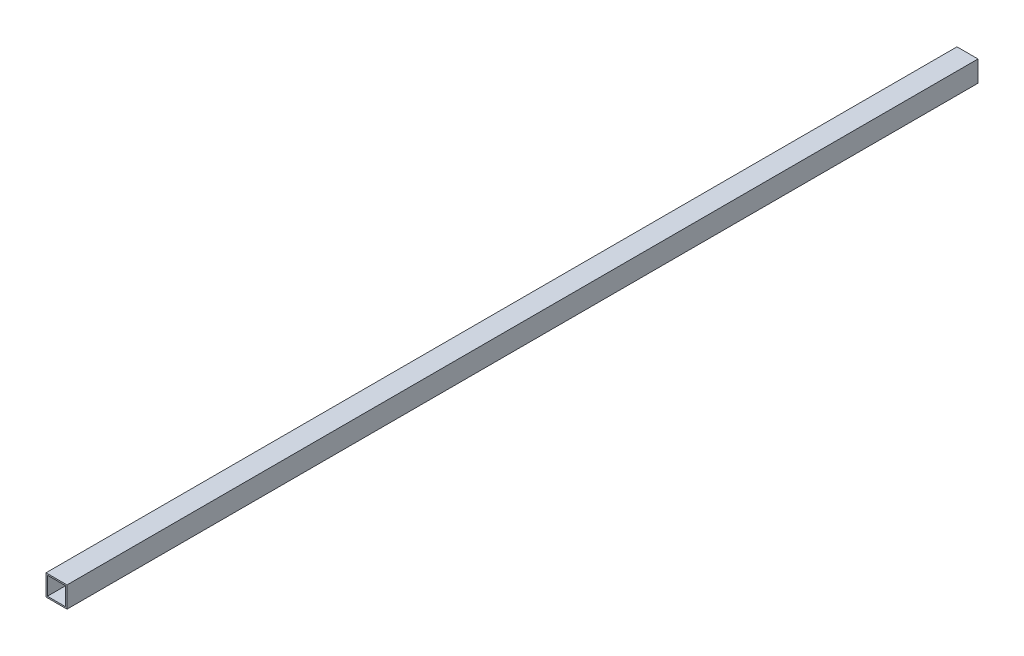
from build123d import *

# Parameters (mm, degrees)
SKETCH_1_W      = 30
SKETCH_1_H      = 30
SKETCH_1_W_2    = 26
SKETCH_1_H_2    = 26
EXTRUDE_1_DEPTH = 650


with BuildPart() as part:
    # 草图1 → 凸台-拉伸1 (new, symmetric)
    with BuildSketch(Plane.XY):
        Rectangle(SKETCH_1_W, SKETCH_1_H)
        Rectangle(SKETCH_1_W_2, SKETCH_1_H_2, mode=Mode.SUBTRACT)
    extrude(amount=EXTRUDE_1_DEPTH, both=True)


solid = part.part
